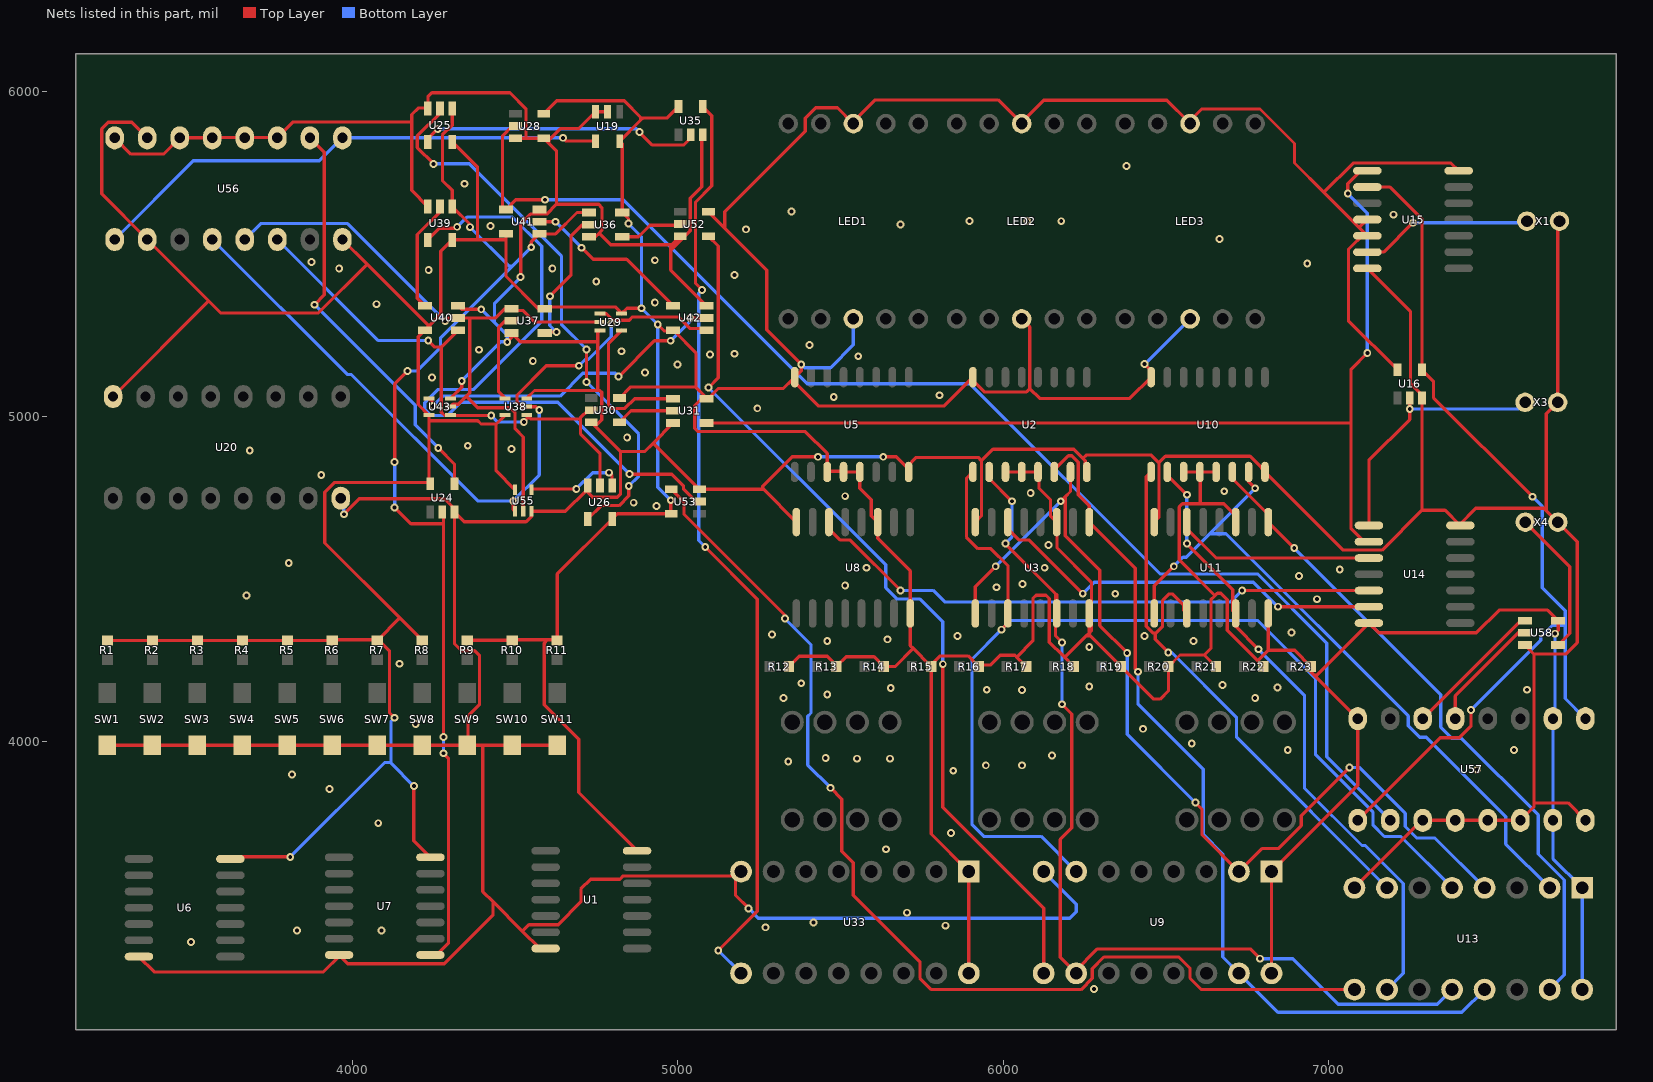
[diagram p0: the nets of this part, all layers, seen from the top]
# Altium PCB MISC50897.pcbdoc (part 2 of 2)
Units mil, origin at the board's own origin, x right, y up, seen from the top; angles counter-clockwise.
Board outline 4735 x 3000 mil, 2 copper layers (Top Layer, Bottom Layer), stack 62.206 mil thick; 82 components, 112 nets, 500 pads, 251 vias.

## Via types
v1: diameter 24.02, hole 12, Top Layer to Bottom Layer, 251 vias

## Nets (pads, with @x,y where several pads share a name; then routed paths per layer and width w, separated by ;. In a path a pad name is that pad's centre, name@x,y a point inside that pad or via, vN(x,y) a via of type N, cw(c..) or ccw(c..) an arc to the next point about the centre after c; other vN are vias at no path point) (continued)
$1N14547: U7.8 U24.2 U25.1 U36.1 U39.1 U41.1 | length 3388.9
  Top Layer w10: v1(4130.37,4720) 4180.37,4670 4280.37,4670 ; v1(4130.37,4860) 4130.37,5100 v1(4170.37,5140) ; U7.8@4240.37,3345 4260.37,3345 4295.73,3380.36 4295.73,3949.64 v1(4280.37,3965) ; U24.2@4276.98,4706.69 4280.37,4703.31 4280.37,4670 ; v1(4280.37,4015) 4280.37,4670 ; U25.1@4307.4,5946.19 4307.4,5895.07 4277.4,5865.07 4277.4,5725.07 4307.4,5695.07 U39.1@4307.4,5645.07 4362.05,5590.42 v1(4362.05,5581.68) ; v1(4550.37,5520) 4550.37,5536.29 U41.1@4575.06,5560.98 4625.06,5560.98 4690.88,5626.8 U36.1@4727.44,5626.8
  Bottom Layer w10: v1(4130.37,4720) v1(4130.37,4860) ; v1(4170.37,5140) 4200.37,5140 4271.08,5210.71 4271.08,5240.71 4492.05,5461.68 ; v1(4280.37,3965) v1(4280.37,4015) ; v1(4362.05,5581.68) 4482.05,5461.68 4492.05,5461.68 ; v1(4550.37,5520) 4492.05,5461.68
$1N14710: U19.4 U56.1 U56.9 | length 1611.2
  Top Layer w10: v1(4647.6,5856.26) 4657.6,5846.26 U19.4@4747.6,5846.26
  Bottom Layer w10: U56.9@3270,5543.7 3511.85,5785.55 3899.33,5785.55 U56.1@3970,5856.3 v1(4647.6,5856.26)
$1N14725: U24.4 U56.2 | length 1271.9
  Top Layer w10: U56.2@3870,5856.3 3914.39,5811.9 3914.39,5373.31 v1(3884.39,5343.31) ; v1(4264.4,4903.31) 4314.4,4853.31 U24.4@4314.4,4793.31
  Bottom Layer w10: v1(3884.39,5343.31) 4193.68,5034.02 4193.68,4974.02 v1(4264.4,4903.31)
$1N14861: U15.2 U16.4 U57.1 U57.9 | length 2873.7
  Top Layer w10: U57.1@7090,3758.7 7343.55,4012.25 7402.76,4012.25 7438.12,4047.6 v1(7438.12,4097.6) ; U15.2@7119.63,5705 7189.63,5705 7287.4,5607.23 U16.4@7287.4,5143.31 7322.76,5107.96 7322.76,5057.96 v1(7627.4,4753.31)
  Bottom Layer w10: v1(7438.12,4097.6) 7652.76,4312.25 7652.76,4322.25 7688.12,4357.6 7728.12,4357.6 ; v1(7627.4,4753.31) 7657.4,4723.31 7657.4,4473.31 7728.12,4402.6 7728.12,4357.6 ; U57.9@7790,4071.3 7728.12,4133.18 7728.12,4357.6
$1N16239: U9.9 U52.4 | length 2757.9
  Top Layer w10: U52.4@5094.79,5553.98 5125,5523.77 5125,5118.7 v1(5095,5088.7) ; v1(5815,4238.7) 5815,3798.7 6125,3488.7 U9.9@6125,3288.7
  Bottom Layer w10: v1(5095,5088.7) 5639.64,4544.06 5639.64,4474.06 5675,4438.7 5745,4438.7 5815,4368.7 v1(5815,4238.7)
$1N16309: U13.9 U53.4 | length 3294.8
  Top Layer w10: U53.4@4980.21,4775.93 5020,4736.14 5020,4698.7 5330,4388.7 v1(5330,4378.7) ; v1(5470,3858.7) 5504.64,3824.06 5504.64,3664.06 5540,3628.7 5540,3528.7 5744.64,3324.06 5744.64,3274.06 5780,3238.7 6240,3238.7 6274.64,3273.34 6274.64,3303.34 6310,3338.7 6540,3338.7 6574.64,3304.06 6574.64,3274.06 6610,3238.7 U13.9@7080,3238.7
  Bottom Layer w10: v1(5330,4378.7) 5410,4298.7 5410,4088.7 5400,4078.7 5400,3928.7 v1(5470,3858.7)
$1N16449: U30.4 U31.2 | length 179.6
  Top Layer w10: U30.4@4821.36,4981.92 4856.78,5017.34 U31.2@4986.31,5017.34
$1N18341: U36.4 U52.2 | length 194.7
  Top Layer w10: U36.4@4829.81,5552 4879.81,5552 4915.16,5587.35 5004.13,5587.35 U52.2@5008.17,5591.39
$1N18345: U39.4 U53.2 | length 2131.6
  Top Layer w10: U39.4@4232.6,5542.7 4267.96,5578.06 4317.96,5578.06 v1(4322.6,5582.7) ; v1(4852.6,4822.7) 4982.6,4822.7 5017.96,4787.35 5017.96,4777.35 5053.31,4741.99 5063.36,4741.99 U53.2@5066.83,4738.52
  Bottom Layer w10: v1(4322.6,5582.7) 4352.6,5612.7 4492.6,5612.7 4582.6,5522.7 4582.6,5292.7 4372.6,5082.7 4262.6,5082.7 4222.6,5042.7 4222.6,5022.7 4242.6,5002.7 4292.6,5002.7 4333.61,5043.72 4631.59,5043.72 v1(4852.6,4822.7)
$1N18742: U57.14 U58.1 | length 438.5
  Top Layer w10: U57.14@7290,4071.3 7591.1,4372.4 U58.1@7603.81,4372.4
$1N18746: U57.13 U58.2 | length 364
  Top Layer w10: U57.13@7390,4071.3 7390,4141.19 7583.81,4335 U58.2@7603.81,4335
$1N18772: U58.4 X4.1 | length 448.6
  Top Layer w10: X4.1@7605,4675 7741.54,4538.46 7741.54,4332.96 U58.4@7706.19,4297.6
$1N18830: U28.2 U41.4 U57.2 | length 4008.1
  Top Layer w10: U28.2@4502.11,5892.5 4492.11,5892.5 4462.11,5862.5 4462.11,5646.35 U41.4@4472.69,5635.78 4502.69,5665.78 v1(4592.69,5665.78)
  Bottom Layer w10: v1(4592.69,5665.78) 4832.69,5665.78 5398.38,5100.09 5898.38,5100.09 6482.69,4515.78 6782.69,4515.78 6994.82,4303.64 6994.82,3953.88 U57.2@7190,3758.7
$1N19160: U33.9 U35.4 | length 2861.4
  Top Layer w10: v1(5075,5388.7) 5055,5408.7 5055,5658.7 5105,5708.7 5105,5924.69 U35.4@5077.4,5952.29 ; v1(5085,4598.7) 5245,4438.7 5245,3478.7 v1(5125,3358.7)
  Bottom Layer w10: v1(5075,5388.7) 5065,5378.7 5065,4618.7 v1(5085,4598.7) ; v1(5125,3358.7) U33.9@5195,3288.7
$1N21103: U25.4 U35.2 | length 869.6
  Top Layer w10: U25.4@4232.6,5843.81 4232.6,5853.81 v1(4262.6,5883.81) ; v1(4882.6,5873.81) 4922.6,5833.81 5018.14,5833.81 5039.99,5855.67 U35.2@5039.99,5865.67
  Bottom Layer w10: v1(4262.6,5883.81) 4872.6,5883.81 v1(4882.6,5873.81)
$1N21118: U25.2 U26.4 | length 1733.2
  Top Layer w10: v1(4250,5776.19) 4200,5826.19 4200,5861.95 4270,5931.95 U25.2@4270,5946.19 ; v1(4720,5106.19) v1(4720,5206.19) ; U26.4@4723.89,4684.84 4765.24,4726.19 4820,4726.19 4850,4756.19 v1(4850,4786.19)
  Bottom Layer w10: v1(4250,5776.19) 4360,5776.19 4642.84,5493.34 4642.84,5283.34 v1(4720,5206.19) ; v1(4720,5106.19) 4880,4946.19 4880,4816.19 v1(4850,4786.19)
$1N21124: U26.2 U30.2 U38.1 U40.1 U43.1 U56.14 | length 1653.9
  Top Layer w10: v1(4233.57,5233.11) 4253.57,5213.11 4273.57,5213.11 ; U43.1@4302.13,5004.25 U43.1@4303.57,5002.82 ; U40.1@4325.67,5265.22 4273.57,5213.11 ; v1(4427.44,5002.82) U43.1@4303.57,5002.82 ; v1(4527.44,4982.82) 4537.44,4992.82 U38.1@4537.44,5002.82 ; U38.1@4536.01,5004.25 U38.1@4537.44,5002.82 ; U30.2@4734.74,5019.33 4724.74,5019.33 4701.29,4995.88 4701.29,4992.21 ; U26.2@4761.29,4787.21 4761.29,4887.21 4701.29,4947.21 4701.29,4992.21 ; 4273.57,5213.11 4273.57,5012.82 4283.57,5002.82 U43.1@4303.57,5002.82 ; U38.1@4537.44,5002.82 4548.05,4992.21 4701.29,4992.21
  Bottom Layer w10: U56.14@3770,5543.7 4080.59,5233.11 v1(4233.57,5233.11) ; v1(4427.44,5002.82) 4447.44,4982.82 v1(4527.44,4982.82)
$1N21143: U26.1 U55.4 | length 303.3
  Top Layer w10: U55.4@4551.26,4774.72 4553.75,4777.21 v1(4688.69,4777.21) ; v1(4788.69,4827.21) 4798.69,4817.21 U26.1@4798.69,4787.21
  Bottom Layer w10: v1(4688.69,4777.21) 4738.69,4827.21 v1(4788.69,4827.21)
$1N21148: U29.2 U37.1 U40.2 U43.2 U55.2 U56.13 | length 2060.2
  Top Layer w10: v1(4285.67,5292.62) 4295.67,5302.62 U40.2@4325.67,5302.62 4361.02,5302.62 ; U43.2@4302.13,5029.85 4309.55,5037.27 4325.67,5037.27 4350.42,5062.01 ; U55.2@4525.67,4708.38 4525.67,4936.76 4500.42,4962.01 4500.42,5012.01 4485.77,5026.66 4385.77,5026.66 4350.42,5062.01 ; U29.2@4761.42,5290.11 4561.42,5290.11 4526.06,5325.46 4495.03,5325.46 U37.1@4489.44,5331.04 4469.44,5331.04 4441.02,5302.62 4361.02,5302.62 ; 4350.42,5062.01 4361.02,5072.62 4361.02,5302.62
  Bottom Layer w10: U56.13@3670,5543.7 3718.92,5592.62 3985.67,5592.62 v1(4285.67,5292.62)
$1N21155: U29.1 U38.2 U42.1 U55.1 U56.12 | length 2479
  Top Layer w10: v1(4494.78,4739.85) 4494.78,4713.67 U55.1@4500.07,4708.38 ; v1(4574.78,5019.85) 4564.78,5029.85 U38.2@4536.01,5029.85 4522.28,5029.85 4506.42,5045.71 4506.42,5065.71 4596.42,5155.71 v1(4696.42,5155.71) ; U29.1@4761.42,5315.71 4781.42,5315.71 4801.42,5295.71 4806.42,5295.71 ; v1(4796.42,5285.71) 4806.42,5295.71 ; U42.1@5088.68,5265.22 5083.55,5270.35 5036.77,5270.35 5001.42,5305.71 4861.42,5305.71 4851.42,5295.71 4806.42,5295.71
  Bottom Layer w10: U56.12@3570,5543.7 3984.49,5129.21 3996.32,5129.21 4385.23,4740.3 v1@4495.23,4740.3 ; v1(4494.78,4739.85) v1@4495.23,4740.3 ; v1(4574.78,5019.85) 4574.78,4819.85 v1@4495.23,4740.3 ; v1(4696.42,5155.71) 4715.71,5175 4725.71,5175 4796.42,5245.71 v1(4796.42,5285.71)
$1N21187: U37.2 U38.4 | length 274.5
  Top Layer w10: U38.4@4469.67,5055.44 4449.67,5075.44 4449.67,5273.64 4469.67,5293.64 U37.2@4489.44,5293.64
$1N21232: U36.2 U37.4 | length 436.6
  Top Layer w10: U37.4@4591.81,5256.24 4594.97,5259.4 v1(4627.44,5259.4) ; v1(4607.44,5369.4) 4672.08,5434.04 4672.08,5554.04 4707.44,5589.4 U36.2@4727.44,5589.4
  Bottom Layer w10: v1(4607.44,5369.4) 4607.44,5279.4 v1(4627.44,5259.4)
$1N21283: U41.2 U42.4 | length 518.3
  Top Layer w10: U41.2@4575.06,5598.38 v1(4625.06,5598.38) ; v1(4705.06,5518.38) 4740.42,5483.02 4843.31,5483.02 U42.4@4986.31,5340.02
  Bottom Layer w10: v1(4625.06,5598.38) v1(4705.06,5518.38)
$1N21292: U42.2 U43.4 | length 994.1
  Top Layer w10: U43.4@4235.79,5055.44 4248.68,5042.55 v1(4248.68,5032.62) ; v1(4818.68,5122.62) 4928.68,5232.62 v1(4978.68,5232.62) ; v1(5038.68,5302.62) U42.2@5088.68,5302.62
  Bottom Layer w10: v1(4248.68,5032.62) 4278.68,5062.62 4638.68,5062.62 4708.68,5132.62 4808.68,5132.62 v1(4818.68,5122.62) ; v1(4978.68,5232.62) 5038.68,5292.62 v1(5038.68,5302.62)
$1N21350: U39.2 U40.4 | length 343.7
  Top Layer w10: U40.4@4223.3,5340.02 4200,5363.32 4200,5559.1 4270,5629.1 U39.2@4270,5645.07
$1N21360: U10.7 U11.9 U13.2 | length 2139.3
  Top Layer w10: U11.9@6465,4394.63 6465,4479.33 v1(6525,4539.33) ; U10.7@6755,4829.33 6755,4799.33 v1(6775,4779.33)
  Bottom Layer w10: v1(6525,4539.33) 6552.87,4567.2 6562.87,4567.2 6635.35,4639.68 ; v1(6775,4779.33) 6635.35,4639.68 ; U13.2@7679.99,3551.3 7545.35,3685.95 7545.35,3769.68 7300.7,4014.32 7280.7,4014.32 7245.35,4049.68 7245.35,4079.68 6685.35,4639.68 6635.35,4639.68
$1N21369: U2.7 U3.9 U9.2 U13.4 | length 3010.7
  Top Layer w10: U3.9@5915,4394.63 5915,4476.83 v1(5977.5,4539.33) ; v1(6177.5,4739.33) 6191.59,4753.42 ; U2.7@6207.5,4829.33 6207.5,4769.33 6191.59,4753.42 ; v1(6381.59,4273.42) 6297.66,4357.36 6297.66,4527.36 6191.59,4633.42 6191.59,4753.42 ; v1(6591.59,3813.42) 6611.59,3793.42 6611.59,3714.71 U9.2@6724.99,3601.3 6795.71,3672.01 6845.71,3672.01 6916.42,3742.72 6916.42,3772.72 v1(7065,3921.3)
  Bottom Layer w10: v1(5977.5,4539.33) v1(6177.5,4739.33) ; v1(6381.59,4273.42) 6381.59,4023.42 v1(6591.59,3813.42) ; v1(7065,3921.3) 7095,3921.3 7236.42,3779.88 7236.42,3739.88 7271.78,3704.52 7326.78,3704.52 U13.4@7479.99,3551.3
$1N21375: U10.1 U11.11 U13.7 | length 1828.4
  Top Layer w10: U10.1@6455,4829.33 6440.3,4814.63 6440.3,4354.63 6460.3,4334.63 6467.8,4334.63 ; v1(6507.8,4274.63) 6467.8,4314.63 6467.8,4334.63 ; U11.11@6565,4394.63 6555.65,4403.98 6555.65,4419.27 6520.3,4454.63 6510.3,4454.63 6490.3,4434.63 6490.3,4354.63 6470.3,4334.63 6467.8,4334.63
  Bottom Layer w10: v1(6507.8,4274.63) 6517.8,4274.63 6717.8,4074.63 6717.8,4013.5 U13.7@7179.99,3551.3
$1N21384: U2.1 U3.11 U9.7 U13.5 | length 3492.1
  Top Layer w10: U2.1@5907.5,4829.33 5887.5,4809.33 5887.5,4629.33 5922.86,4593.98 5962.86,4593.98 6015,4541.83 U3.11@6015,4394.63 6015,4364.63 v1(5995,4344.63)
  Bottom Layer w10: U9.7@6224.99,3601.3 6117.03,3709.27 5940.36,3709.27 5905,3744.63 5905,4254.63 v1(5995,4344.63) 6023.23,4372.86 6783.23,4372.86 6960.01,4196.09 6960.01,3961.29 7136.79,3784.51 7136.79,3744.51 7172.14,3709.16 7222.14,3709.16 U13.5@7379.99,3551.3
$1N21390: U10.2 U11.14 U13.10 | length 1917.5
  Top Layer w10: U10.2@6505,4829.33 6505,4819.33 v1(6565,4759.33) ; v1(6565,4609.33) 6706.42,4467.91 6706.42,4403.21 U11.14@6715,4394.63 6715,4354.63 v1(6785,4284.63)
  Bottom Layer w10: v1(6565,4609.33) v1(6565,4759.33) ; v1(6785,4284.63) 6926.42,4143.21 6926.42,3858.21 7103.2,3681.43 7113.2,3681.43 7230,3564.63 7230,3288.7 U13.10@7180,3238.7
$1N21399: U2.2 U3.14 U9.10 U13.12 | length 3037.7
  Top Layer w10: U2.2@5957.5,4829.33 5957.5,4809.33 v1(6027.5,4739.33) ; v1(6007.5,4609.33) 6161.3,4455.54 ; U3.14@6165,4394.63 6165,4451.83 6161.3,4455.54 ; v1(6181.3,4115.54) 6211.3,4085.54 6211.3,3735.54 6175.94,3700.18 6175.94,3337.76 U9.10@6220.14,3293.56 ; v1(6181.3,4305.54) 6161.3,4325.54 6161.3,4455.54 ; U9.10@6225,3288.7 U9.10@6220.14,3293.56 ; v1(6790.14,3333.56) 6760.14,3363.56 6290.14,3363.56 U9.10@6220.14,3293.56
  Bottom Layer w10: v1(6007.5,4609.33) 6027.5,4629.33 v1(6027.5,4739.33) ; v1(6181.3,4115.54) v1(6181.3,4305.54) ; v1(6790.14,3333.56) 6890.14,3333.56 7030.14,3193.56 7334.86,3193.56 U13.12@7380,3238.7
$1N21405: U10.6 U11.1 U13.15 | length 2049.3
  Top Layer w10: U10.6@6705,4829.33 6705,4809.33 6811.07,4703.27 6811.07,4679.3 U11.1@6815,4675.37 v1(6895,4595.37)
  Bottom Layer w10: v1(6895,4595.37) 7345,4145.37 7345,4045.37 7380.36,4010.01 7410.36,4010.01 7645,3775.37 7645,3655.37 7725,3575.37 7725,3283.7 U13.15@7680,3238.7
$1N21413: U2.6 U3.1 U9.15 U13.13 | length 2715.3
  Top Layer w10: U2.6@6157.5,4829.33 6157.5,4835.8 6201.04,4879.33 6211.04,4879.33 6231.04,4859.33 6231.04,4759.33 6265,4725.37 U3.1@6265,4675.37 6406.42,4533.95 6406.42,4223.95 v1(6415,4215.37)
  Bottom Layer w10: v1(6415,4215.37) 6415,4115.37 6615,3915.37 6615,3715.37 6675,3655.37 6675,3338.7 U9.15@6725,3288.7 6845,3168.7 7410,3168.7 U13.13@7480,3238.7
$1N21792: U14.9 U15.1 U31.4 | length 3234.6
  Top Layer w10: U31.4@5088.75,4980 7069.63,4980 ; v1(7059.63,5685) 7059.63,5715 7094.99,5750.36 7114.99,5750.36 U15.1@7119.63,5755 ; v1(7119.63,5195) 7069.63,5145 7069.63,4980 ; U14.9@7124.63,4615 7109.63,4615 7069.63,4655 7069.63,4980
  Bottom Layer w10: v1(7059.63,5685) 7119.63,5625 v1(7119.63,5195)
$1N21809: U11.6 U14.10 | length 617.1
  Top Layer w10: U11.6@6565,4675.37 6565,4655.37 6655.37,4565 U14.10@7124.63,4565
$1N21815: U8.6 U14.12 | length 1787.8
  Top Layer w10: U8.6@5465,4675.37 5465,4655.37 5500.36,4620.01 5530.36,4620.01 v1(5685,4465.37) ; v1(6735,4465.37) 7124.26,4465.37 U14.12@7124.63,4465
  Bottom Layer w10: v1(5685,4465.37) 5785,4465.37 5820.36,4430.01 6699.64,4430.01 v1(6735,4465.37)
$1N21823: U3.6 U14.13 | length 1258.5
  Top Layer w10: U3.6@6015,4675.37 6015,4655.37 6050.36,4620.01 6080.36,4620.01 v1(6245,4455.37) ; v1(6845,4415.37) 7124.26,4415.37 U14.13@7124.63,4415
  Bottom Layer w10: v1(6245,4455.37) 6280.36,4490.73 6769.64,4490.73 v1(6845,4415.37)
$1N21835: U14.8 U16.2 X3.1 | length 806.8
  Top Layer w10: U14.8@7124.63,4665 7124.63,4865 7249.99,4990.36 v1(7249.99,5022.86) U16.2@7249.99,5056.69
  Bottom Layer w10: v1(7249.99,5022.86) 7584.13,5022.86 X3.1@7604.69,5043.42
$1N22185: U29.4 U31.1 | length 461.5
  Top Layer w10: U29.4@4827.76,5264.52 4787.76,5224.52 4787.76,5034.74 4797.76,5024.74 4837.76,5024.74 4867.76,5054.74 U31.1@4986.31,5054.74
$1N23026: U15.6 X1.1 | length 529.7
  Top Layer w10: U15.6@7119.63,5505 7169.63,5505 v1(7259.63,5595)
  Bottom Layer w10: v1(7259.63,5595) 7605,5595 X1.1@7610,5600
GND: SW1.1 SW2.1 SW3.1 SW4.1 SW5.1 SW6.1 SW7.1 SW8.1 SW9.1 SW10.1 SW11.2 U1.7 U2.8 U3.8 U5.8 U6.7 U7.7 U8.8 U9.8 U10.8 U11.8 U13.8 U14.7 U15.7 U16.3 U19.2 U19.3 U20.8 U24.3 U25.3 U26.3 U28.3 U28.4 U29.3 U30.3 U31.3 U33.8 U35.3 U36.3 U37.3 U38.3 U39.3 U40.3 U41.3 U42.3 U43.3 U52.3 U53.3 U55.3 U56.3 U56.4 U56.5 U56.6 U56.8 U57.3 U57.4 U57.5 U57.6 U57.8 U58.3 X1.2 X3.2 X4.2 | length 20390.6
  Top Layer w10: SW1.1@3247.53,3989.88 SW2.1@3385.78,3989.88 SW3.1@3524.02,3989.88 SW4.1@3662.27,3989.88 SW5.1@3800.52,3989.88 SW6.1@3938.77,3989.88 SW7.1@4077.01,3989.88 SW8.1@4215.26,3989.88 SW9.1@4353.51,3989.88 SW9.1@4356.01,3989.88 ; U56.8@3270,5856.3 3320,5806.3 3420,5806.3 U56.6@3470,5856.3 U56.5@3570,5856.3 3571.02,5857.32 U56.4@3671.02,5857.32 ; U6.7@3344.63,3340 3391.82,3292.81 3911.82,3292.81 U7.7@3961.82,3342.81 ; U56.4@3670,5856.3 U56.4@3671.02,5857.32 ; U56.3@3770,5856.3 U56.3@3771.02,5857.32 ; U7.7@3959.63,3345 U7.7@3961.82,3342.81 ; v1(3974.39,4699.31) 4021.76,4746.69 4284.39,4746.69 4314.39,4716.69 U24.3@4314.39,4706.69 ; U39.3@4232.6,5645.07 4182.6,5695.07 4182.6,5902.4 ; U25.3@4232.6,5946.19 U25.3@4232.6,5947.55 ; U43.3@4302.13,5055.44 4336.53,5089.84 v1(4336.53,5109.16) ; U40.3@4325.67,5340.02 4336.54,5329.16 v1(4396.53,5329.16) ; v1(4476.53,5229.16) U37.3@4496.53,5249.16 ; U37.3@4489.44,5256.24 U37.3@4496.53,5249.16 ; U28.3@4502.11,5855.1 4533.73,5855.09 ; v1(4517.64,5428.05) 4517.64,5592 4547.64,5622 4575.14,5622 ; U38.3@4536.01,5055.44 4560.28,5079.71 4754.46,5079.71 ; U41.3@4575.14,5635.7 4575.14,5622 ; U1.7@4594.63,3365 4575.89,3365 4522.98,3417.9 ; SW11.2@4630,3989.88 SW10.1@4491.75,3989.88 4401.01,3989.88 ; U26.3@4723.89,4787.21 4723.89,4777.21 U26.3@4718.7,4772.02 ; U36.3@4727.44,5552 4747.44,5552 4758.6,5563.16 ; U30.3@4734.74,4981.93 4746.96,4969.71 ; U29.3@4761.42,5264.52 4754.46,5257.56 4754.46,5229.71 ; U19.2@4785,5936.62 U19.3@4747.6,5936.62 4695.5,5884.52 4640.02,5884.52 4604.66,5849.17 4604.66,5839.17 ; U31.3@4986.31,4979.94 4923.06,4916.68 ; U52.3@5008.17,5553.99 4981.98,5527.8 4978.95,5527.8 ; U35.3@5077.4,5865.67 5074.31,5862.58 5074.31,5705.66 5038.95,5670.3 5038.95,5570.3 4978.95,5510.3 ; U42.3@5088.68,5340.02 4978.95,5449.75 4978.95,5510.3 ; U33.8@5194.99,3601.3 5181.6,3587.9 U33.8@5177.98,3587.9 ; v1(5217.98,3487.9) 5177.98,3527.9 U33.8@5177.98,3587.9 ; U8.8@5365,4675.37 5264.45,4775.92 5261.83,4775.92 ; v1(5431.83,4875.92) 5351.83,4875.92 5261.83,4785.92 5261.83,4775.92 ; v1(5631.83,4875.92) 5671.83,4875.92 U5.8@5703.65,4844.1 ; U5.8@5710,4829.33 5707.19,4832.15 5707.19,4840.57 U5.8@5703.65,4844.1 ; U3.8@5915,4675.37 5933.65,4694.02 5933.65,4864.1 ; U2.8@6257.5,4829.33 6252.73,4834.1 6252.73,4864.1 6245.66,4871.17 ; U11.8@6465,4675.37 6479.2,4689.57 6479.2,4857.64 ; U13.8@7079.99,3551.3 7287.4,3758.7 U57.3@7290,3758.7 U57.4@7390,3758.7 U57.5@7490,3758.7 U57.6@7590,3758.7 7631.77,3800.47 7631.77,3812.14 ; U15.7@7119.63,5455 7252.04,5322.59 7252.04,5102.05 7287.4,5066.69 U16.3@7287.4,5056.69 7287.4,4711.73 ; U14.7@7405.37,4665 U14.7@7402.84,4667.53 ; U58.3@7603.81,4297.6 7631.77,4269.64 ; X1.2@7710,5600 7704.69,5594.69 X3.2@7704.69,5043.42 7669.54,5008.27 7669.54,4710.46 ; U57.8@7790,3758.7 7736.56,3812.14 7631.77,3812.14 ; U56.4@3671.02,5857.32 U56.3@3771.02,5857.32 ; U56.3@3771.02,5857.32 3818.75,5905.05 4179.95,5905.05 4182.6,5902.4 ; U7.7@3961.82,3342.81 3986.57,3318.06 4282.83,3318.06 4432.83,3468.06 4432.83,3508.06 ; 4182.6,5902.4 4182.6,5927.83 4202.32,5947.55 U25.3@4232.6,5947.55 ; U25.3@4232.6,5947.55 4232.6,5982.6 4245,5995 4484.92,5995 4533.73,5946.19 4533.73,5855.09 ; U24.3@4314.39,4706.69 4314.39,4301.5 4336.01,4279.88 4376.01,4279.88 4391.36,4264.52 4391.36,4115.24 4356.01,4079.88 SW9.1@4356.01,3989.88 ; U24.3@4314.39,4706.69 4344.39,4676.69 4534.39,4676.69 4551.26,4693.57 U55.3@4551.26,4708.38 4655.06,4708.38 U26.3@4718.7,4772.02 ; SW9.1@4356.01,3989.88 4401.01,3989.88 ; 4401.01,3989.88 4401.01,3539.88 4432.83,3508.06 ; 4432.83,3508.06 4522.98,3417.9 ; U37.3@4496.53,5249.16 4515.98,5229.71 4754.46,5229.71 ; 4522.98,3417.9 4542.98,3437.9 4632.98,3437.9 4702.98,3507.9 4702.98,3547.9 4732.98,3577.9 4822.98,3577.9 4832.98,3587.9 U33.8@5177.98,3587.9 ; 4533.73,5855.09 U28.4@4588.73,5855.09 4604.66,5839.17 ; 4575.14,5622 4597.64,5622 4627.64,5652 ; 4604.66,5839.17 4627.64,5816.19 4627.64,5652 ; 4627.64,5652 4757.44,5652 4767.44,5642 4767.44,5572 4758.6,5563.16 ; U26.3@4718.7,4772.02 4738.7,4752.02 4814.74,4752.02 4824.74,4762.02 4824.74,4891.93 ; 4746.96,4969.71 4766.96,4989.71 4766.96,5073.95 4761.2,5079.71 4754.46,5079.71 ; 4746.96,4969.71 4824.74,4891.93 ; 4754.46,5079.71 4754.46,5229.71 ; 4758.6,5563.16 4793.95,5527.8 4978.95,5527.8 ; 4824.74,4891.93 4898.31,4891.93 4923.06,4916.68 ; 4923.06,4916.68 4926.08,4916.68 U53.3@5066.83,4775.92 5261.83,4775.92 ; 4978.95,5510.3 4978.95,5527.8 ; U5.8@5703.65,4844.1 5733.65,4874.1 5923.65,4874.1 5933.65,4864.1 ; 5933.65,4864.1 5969.01,4899.46 6217.38,4899.46 6245.66,4871.17 ; 6245.66,4871.17 6255.66,4881.17 6455.66,4881.17 6479.2,4857.64 ; 6479.2,4857.64 6499.2,4877.64 6759.2,4877.64 6794.55,4842.28 6794.55,4839.78 U10.8@6805,4829.33 7045,4589.33 7165,4589.33 7287.4,4711.73 ; 7287.4,4711.73 7358.64,4711.73 U14.7@7402.84,4667.53 ; U14.7@7402.84,4667.53 7452.84,4717.53 7662.47,4717.53 7669.54,4710.46 ; 7631.77,3812.14 7631.77,4269.64 ; 7631.77,4269.64 7729.64,4269.64 7765,4305 7765,4615 X4.2@7705,4675 7669.54,4710.46
  Bottom Layer w10: U20.8@3965,4748.7 3974.39,4739.31 v1(3974.39,4699.31) ; v1(4336.53,5109.16) 4456.53,5229.16 v1(4476.53,5229.16) 4476.53,5249.16 4437.64,5288.05 ; v1(4396.53,5329.16) 4437.64,5288.05 ; v1(4517.64,5428.05) 4437.64,5348.05 4437.64,5288.05 ; v1(5217.98,3487.9) 5247.98,3457.9 6205,3457.9 6225,3477.9 6225,3501.3 U9.8@6124.99,3601.3 ; v1(5431.83,4875.92) v1(5631.83,4875.92)
  other v1: 6280,3240 3505,3385 3830,3420 4090,3420 5270,3430 5823.4,3435 5417.63,3445 5705,3475 5640,3670 5840,3720 4080,3750 3930,3855 3815,3900 5847.16,3911.13 7456.4,3915 5947.25,3927.78 6058.71,3927.78 5340,3940 5551.07,3948.29 5652.43,3948.29 5455,3950 6150.86,3957.6 6875,3975 7570,3975 6580,3995 6430,4040 4195,4055 5325,4135 6775,4135 5460,4145 6058.3,4158.97 5950,4160 7610,4160 5655,4165 6843.56,4166.57 6265,4170 6675,4175 5380,4180 4145,4240 6265,4291.54 5460,4310 6585,4310 5645,4315 5860,4325 6435,4325 5290,4330 6886.43,4336.2 6965,4438.36 3675,4450 6345,4455 5980,4475 5515,4480 6060,4485 6910,4510 7035,4530 5580.21,4535 6128.03,4535 3805,4550 6140,4605 4935,4725 4865,4735 5515,4755 6085,4765 6680,4770 3905,4820 3685,4895 4490,4900 4355,4910 4845,4935 5245,5025 5480,5060 5805,5065 4245,5120 4900,5135 5000,5160 4555,5170 5555,5185 5100,5190 5175,5192.52 4827.76,5200.42 4390,5205 5405,5220 4075,5345 4930,5350 4750,5415 5175,5435 4235,5450 3960,5455 4615,5455 6935,5470 3875,5475 4930,5480 6665,5545 5210,5575 4425,5585 5685,5590 6178.88,5600 5897.08,5600.53 6074.42,5600.53 7200,5620 5350,5630 4345,5715 6380,5770
VCC: LED1.3 LED1.8 LED2.3 LED2.8 LED3.3 LED3.8 R1.2 R2.2 R3.2 R4.2 R5.2 R6.2 R7.2 R8.2 R9.2 R10.2 R11.2 R12.2 R13.2 R14.2 R15.2 R16.2 R17.2 R18.2 R19.2 R20.2 R21.2 R22.2 R23.2 U1.14 U2.3 U2.4 U2.5 U2.16 U3.3 U3.16 U5.3 U5.4 U5.5 U5.16 U6.14 U7.14 U8.3 U8.16 U9.1 U9.16 U10.3 U10.4 U10.5 U10.16 U11.3 U11.16 U13.1 U13.16 U14.14 U15.4 U15.5 U15.14 U16.5 U19.5 U20.16 U24.5 U25.5 U26.5 U28.5 U29.5 U30.5 U31.5 U33.1 U33.16 U35.5 U36.5 U37.5 U38.5 U39.5 U40.5 U41.5 U42.5 U43.5 U52.5 U53.5 U55.5 U56.7 U56.10 U56.16 U57.7 U57.10 U57.16 U58.5 | length 28082.1
  Top Layer w10: R1.2@3247.53,4311.55 R2.2@3385.78,4311.55 R3.2@3524.02,4311.55 R4.2@3662.27,4311.55 R5.2@3800.52,4311.55 R6.2@3938.77,4311.55 3941.25,4314.03 R7.2@4079.49,4314.03 ; U20.16@3265,5061.3 3558.68,5354.98 ; U56.7@3370,5856.3 3322.6,5903.7 3250,5903.7 3230,5883.7 3230,5683.7 U56.10@3370,5543.7 3595.8,5317.9 3895.8,5317.9 4045.8,5467.9 ; U6.14@3625.37,3640 3631.9,3646.53 v1(3809.49,3646.53) ; U56.16@3970,5543.7 4045.8,5467.9 ; R7.2@4077.01,4311.55 R7.2@4079.49,4314.03 ; v1(4129.49,4074.03) 4114.85,4088.68 4114.85,4278.68 R7.2@4079.49,4314.03 ; v1(4189.49,3864.03) 4189.49,3695.88 U7.14@4240.37,3645 ; R8.2@4215.26,4311.55 4149.14,4377.67 ; U24.5@4239.59,4793.31 U24.5@4235.79,4797.1 ; U25.5@4307.4,5843.81 4385.19,5766.02 4385.19,5542.67 ; R9.2@4353.51,4311.55 4353.84,4311.88 R10.2@4492.08,4311.88 ; U38.5@4469.67,5004.25 4442.17,4976.75 ; U41.5@4472.69,5560.98 4472.69,5542.67 ; R10.2@4491.75,4311.55 R10.2@4492.08,4311.88 ; U55.5@4500.07,4774.72 4442.17,4832.62 4442.17,4976.75 ; U28.5@4588.73,5929.9 4628.73,5969.9 4836.04,5969.9 4886.04,5919.9 4886.04,5909.9 ; R11.2@4630,4311.55 R11.2@4630,4313.65 ; U30.5@4821.36,5056.73 4854.73,5090.09 5056.21,5090.09 ; U29.5@4827.76,5315.71 U29.5@4828.64,5316.59 ; v1(4849.03,5592.5) 4849.03,5607.57 U36.5@4829.81,5626.8 4829.81,5838.85 U19.5@4822.4,5846.26 4886.04,5909.9 ; U1.14@4875.37,3665 4696.07,3844.3 4696.07,4007.58 4590,4113.65 4590,4303.65 4600,4313.65 ; v1(4889.03,5332.5) 4844.55,5332.5 U29.5@4828.64,5316.59 ; v1(4939.03,5282.5) 4959.03,5262.5 U42.5@4989.03,5262.5 ; v1(4979.03,4742.5) 4979.03,4702.3 U53.5@4980.21,4701.12 4814.97,4701.12 U26.5@4798.69,4684.84 4630,4516.15 R11.2@4630,4313.65 ; U42.5@4986.31,5265.22 U42.5@4989.03,5262.5 ; U35.5@5002.6,5952.29 4967.28,5916.97 4893.11,5916.97 4886.04,5909.9 ; U31.5@5088.68,5054.74 U31.5@5091.57,5054.74 ; U52.5@5094.79,5628.79 5144.89,5578.69 ; R12.2@5342.09,4231.43 5373.8,4263.15 5459.62,4263.15 R13.2@5489.62,4233.15 ; U5.3@5460,4829.33 U5.3@5460,4831.3 ; R13.2@5487.91,4231.43 R13.2@5489.62,4233.15 ; LED1.8@5540,5900 LED1.8@5537.27,5902.73 ; U33.16@5895,3288.7 U33.1@5895,3601.3 5779.54,3716.76 R15.2@5779.54,4231.43 R15.2@5776.87,4234.1 ; U2.16@5907.5,5120.67 U2.16@5902.3,5115.47 ; R16.2@5925.36,4231.43 R16.2@5920.97,4235.82 ; U2.3@6007.5,4829.33 U2.4@6057.5,4829.33 U2.5@6107.5,4829.33 6110.28,4826.56 6110.28,4780.09 6145.63,4744.74 6145.63,4694.74 6165.63,4674.74 6165.63,4597.15 6271.7,4491.08 6271.7,4341.08 6265,4334.39 ; LED2.3@6057.5,5300 6082.3,5275.2 6082.3,5085.47 ; LED2.8@6057.5,5900 LED2.8@6055.48,5902.02 ; R17.2@6071.18,4231.43 6042.1,4260.52 ; R18.2@6217,4231.43 6184.52,4263.91 ; U3.16@6265,4394.63 6265,4334.39 ; v1(6435,5160.67) 6455,5140.67 U10.16@6455,5120.67 6389.8,5055.47 6112.3,5055.47 6082.3,5085.47 ; U10.3@6555,4829.33 U10.4@6605,4829.33 ; LED3.8@6575,5900 LED3.8@6570.16,5904.84 ; R21.2@6654.45,4231.43 6619.1,4266.79 ; U10.5@6655,4829.33 U10.4@6605,4829.33 ; U11.3@6715,4675.37 6713.89,4676.48 6713.89,4696.48 6678.53,4731.84 6606.47,4731.84 ; R22.2@6800.27,4231.43 6782.79,4248.91 ; U11.16@6815,4394.63 6815,4281.13 ; U9.16@6825,3288.7 U9.1@6825,3601.3 7090,3866.3 U57.16@7090,4071.3 6956.69,4204.61 ; U15.5@7119.63,5555 U15.5@7111.52,5563.11 ; U15.4@7119.63,5605 7095.42,5580.79 7093.84,5580.79 ; U16.5@7212.6,5143.31 7061.52,5294.39 7061.52,5513.11 U15.5@7111.52,5563.11 ; U15.14@7400.37,5755 7376.75,5778.62 7076.01,5778.62 6986.01,5688.62 ; v1(7696.19,4332.4) 7706.19,4342.4 U58.5@7706.19,4372.4 7673.59,4405 7524.63,4405 7454.63,4335 7154.63,4335 U14.14@7124.63,4365 6964.24,4204.61 6956.69,4204.61 ; 4045.8,5467.9 4234.96,5278.74 U40.5@4234.96,5276.87 ; R7.2@4079.49,4314.03 4143.13,4377.67 4149.14,4377.67 ; 4149.14,4377.67 3915.79,4611.02 3915.79,4767.1 3945.79,4797.1 U24.5@4235.79,4797.1 ; U40.5@4234.96,5276.87 4272.08,5314 4272.08,5507.31 U39.5@4307.4,5542.7 4385.19,5542.67 ; U40.5@4234.96,5276.87 U40.5@4223.3,5265.22 4203.3,5245.22 4203.3,5036.74 U43.5@4235.79,5004.25 4235.79,4986.75 ; U24.5@4235.79,4797.1 4235.79,4986.75 ; 4235.79,4986.75 4385.79,4986.75 4395.79,4976.75 4442.17,4976.75 ; 4385.19,5542.67 4472.69,5542.67 ; 4472.69,5542.67 4472.69,5430.17 4571.81,5331.04 U37.5@4591.81,5331.04 4597.36,5336.59 4808.64,5336.59 U29.5@4828.64,5316.59 ; R10.2@4492.08,4311.88 4493.85,4313.65 4600,4313.65 ; 4600,4313.65 R11.2@4630,4313.65 ; U42.5@4989.03,5262.5 5056.21,5195.33 5056.21,5090.09 ; 5056.21,5090.09 U31.5@5082.73,5063.58 ; U31.5@5082.73,5063.58 5052.73,5033.58 5052.73,4963.58 5062.73,4953.58 5392.73,4953.58 5460,4886.3 U5.3@5460,4831.3 ; U31.5@5082.73,5063.58 U31.5@5091.57,5054.74 ; U31.5@5091.57,5054.74 5094.07,5054.74 5125.2,5085.87 5325.2,5085.87 U5.16@5351.72,5112.39 ; 5144.89,5578.69 5144.89,5628.69 5392.37,5876.18 5392.37,5916.18 5424.89,5948.69 5491.31,5948.69 LED1.8@5537.27,5902.73 ; 5144.89,5578.69 5273.93,5449.64 5273.93,5266.07 v1(5380,5160) 5380,5140.67 U5.16@5360,5120.67 U5.16@5351.72,5112.39 ; U5.16@5351.72,5112.39 5431.72,5032.39 5819.22,5032.39 U2.16@5902.3,5115.47 ; U5.3@5460,4831.3 5508.03,4831.3 U5.4@5510,4829.33 U5.5@5560,4829.33 5560,4779.33 5595.36,4743.98 5595.36,4695.01 U8.3@5615,4675.37 5615,4625.37 5715,4525.37 U8.16@5715,4394.63 5715,4295.98 5723.84,4287.14 ; R13.2@5489.62,4233.15 5517.91,4261.43 5603.72,4261.43 R14.2@5633.72,4231.43 5668.14,4231.43 5723.84,4287.14 ; LED1.8@5537.27,5902.73 5607.27,5972.73 5984.77,5972.73 LED2.8@6055.48,5902.02 ; 5723.84,4287.14 R15.2@5776.87,4234.1 ; R15.2@5776.87,4234.1 5806.87,4264.1 5892.69,4264.1 R16.2@5920.97,4235.82 ; U2.16@5902.3,5115.47 5942.3,5075.47 6072.3,5075.47 6082.3,5085.47 ; R16.2@5920.97,4235.82 5960.97,4235.82 5990.97,4265.82 6036.79,4265.82 6042.1,4260.52 ; 6042.1,4260.52 6092.1,4310.52 6092.1,4440.52 6102.1,4450.52 6132.1,4450.52 6142.1,4440.52 6142.1,4306.33 6184.52,4263.91 ; LED2.8@6055.48,5902.02 6125.48,5972.02 6502.98,5972.02 LED3.8@6570.16,5904.84 ; 6184.52,4263.91 6194.52,4263.91 6256.39,4325.78 ; 6256.39,4325.78 6268.47,4325.78 R19.2@6362.81,4231.43 6462.81,4131.43 6482.81,4131.43 6508.63,4157.25 R20.2@6508.63,4231.43 6543.99,4266.79 6619.1,4266.79 ; 6256.39,4325.78 6265,4334.39 ; LED3.8@6570.16,5904.84 6610.16,5944.84 6789.79,5944.84 6895.85,5838.78 6895.85,5778.78 6986.01,5688.62 ; U10.4@6605,4829.33 6606.47,4827.86 6606.47,4731.84 ; 6606.47,4731.84 6551.47,4731.84 6541.47,4721.84 6541.47,4559.16 6651.47,4449.16 ; 6619.1,4266.79 6639.1,4286.79 6639.1,4436.79 6651.47,4449.16 ; 6651.47,4449.16 6659.1,4456.79 6669.1,4456.79 6689.1,4436.79 6689.1,4342.61 6782.79,4248.91 ; 6782.79,4248.91 6815,4281.13 ; 6815,4281.13 6896.39,4281.13 R23.2@6946.09,4231.43 6946.09,4215.21 6956.69,4204.61 ; 6986.01,5688.62 7093.84,5580.79 ; 7093.84,5580.79 U15.5@7111.52,5563.11
  Bottom Layer w10: v1(3809.49,3646.53) 4099.49,3936.53 4119.49,3936.53 ; v1(4129.49,4074.03) 4119.49,4064.03 4119.49,3936.53 ; v1(4189.49,3864.03) 4119.49,3934.03 4119.49,3936.53 ; v1(4849.03,5592.5) 4889.03,5552.5 v1(4889.03,5332.5) v1(4939.03,5282.5) 4939.03,4782.5 v1(4979.03,4742.5) ; v1(5380,5160) 5390,5150 5470,5150 5540,5220 LED1.3@5540,5300 ; v1(6435,5160.67) 6435.67,5160.67 LED3.3@6575,5300 ; v1(7696.19,4332.4) 7696.19,4077.49 U57.10@7690,4071.3 U57.7@7690,3758.7 7690,3641.3 U13.1@7780,3551.3 U13.16@7780,3238.7
pads on no net: LED1.5 LED2.5 LED3.5 U1.10 U1.11 U1.12 U1.13 U3.2 U3.4 U3.5 U3.7 U6.3 U6.11 U7.1 U7.2 U7.3 U7.4 U7.5 U7.6 U7.11 U8.2 U8.4 U8.5 U8.7 U9.3 U9.6 U9.11 U9.14 U11.2 U11.4 U11.5 U11.7 U13.3 U13.6 U13.11 U13.14 U14.1 U14.2 U14.3 U14.4 U14.5 U14.6 U14.11 U15.3 U15.8 U15.9 U15.10 U15.11 U15.12 U15.13 U16.1 U20.15 U24.1 U28.1 U30.1 U33.3 U33.6 U33.11 U33.14 U35.1 U52.1 U53.1 U56.11 U56.15 U57.11 U57.12 U57.15

## Polygon pours and split planes (outlines as drawn)
GND on Top Layer (solid, remove dead copper, pour order 0): 3000,6300 3000,3000 7995,3000 7995,6300
GND on Bottom Layer (solid, remove dead copper, pour order 2): 3080,6375 3080,3135 8145,3135 8145,6375

## Keep-outs
Board Outline Layer:
  the board outline again, w10

## Other copper
Top Layer:
  drawing of 641 lines, arcs and shapes, not listed
Bottom Layer:
  drawing of 224 lines, arcs and shapes, not listed